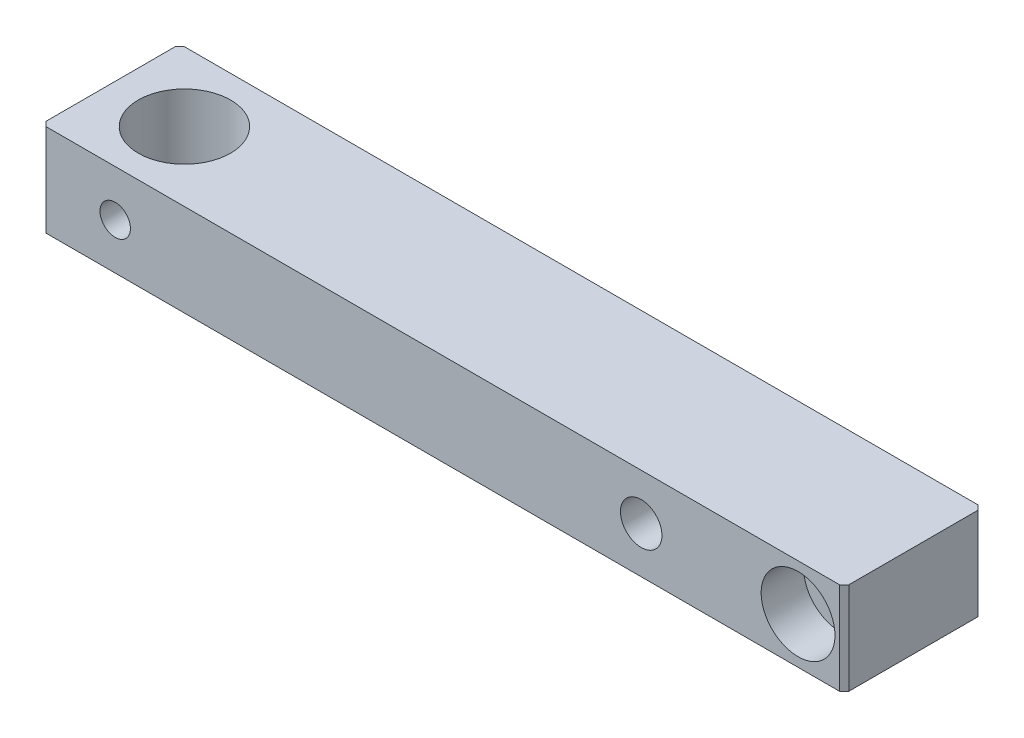
SolidWorks part; units mm, degrees
ref_plane "Front Plane" through (0, 0, 0) normal (0, 0, 1) x (1, 0, 0)
ref_plane "Top Plane" through (0, 0, 0) normal (0, 1, 0) x (1, 0, 0)
ref_plane "Right Plane" through (0, 0, 0) normal (1, 0, 0) x (0, 0, -1)
other "Configuration Table"
sketch "Sketch1" plane through (0, 0, 0) normal (0, 1, 0) x (1, 0, 0)
  line L1 (-43.5, 7.5) -> (43.5, 7.5)
  line L2 (-43.5, 7.5) -> (-43.5, -7.5)
  line L3 (-43.5, -7.5) -> (43.5, -7.5)
  line L4 (43.5, 7.5) -> (43.5, -7.5)
  line L5 (-43.5, 7.5) -> (43.5, -7.5) construction
  line L6 (-43.5, -7.5) -> (43.5, 7.5) construction
  point P0 (0, 0)
  dimension "D1" = 87
  dimension "D2" = 15
extrude "Boss-Extrude1" add sketch "Sketch1" along normal blind 10 contours L1 L4 L3 L2
sketch "Sketch2" plane through (0, 10, 0) normal (0, 1, 0) x (1, 0, 0)
  line L0 (-43.5, 7.5) -> (-43.5, -7.5) construction
  circle A0 centre (-35.5, 0) radius 5
  point P4 (-43.5, 0)
  dimension "D1" = 10
  dimension "D2" = 8
extrude "Cut-Extrude1" cut sketch "Sketch2" against normal through all
sketch "Sketch3" plane through (0, 0, -7.5) normal (0, 0, -1) x (-1, 0, 0)
  line L0 (-43.5, 10) -> (-43.5, 0) construction
  point P0 (-38.5, 5)
  point P3 (-43.5, 5)
  dimension "D1" = 5
sketch "Sketch5" plane through (0, 0, -7.5) normal (0, 0, -1) x (-1, 0, 0)
  line L0 (-43.5, 10) -> (-43.5, 0) construction
  point P0 (-21.5, 5)
  point P3 (-43.5, 5)
  dimension "D1" = 22
hole_wizard "Ø4.5 (4.5) Diameter Hole2" positions "Sketch5" profile "Sketch6" hole size "Ø4.5" standard "GB" end condition through all
sketch "Sketch6" plane through (21.5, 5, -7.5) normal (1, 0, 0) x (0, 1, 0)
  line L0 (0, 0) -> (0, 15)
  line L1 (0, 15) -> (2.25, 15)
  line L2 (2.25, 15) -> (2.25, 0)
  line L5 (2.25, 0) -> (0, 0)
  line L11 (0, -6.35) -> (0, 107.95) construction
  dimension "通孔孔直径" = 4.5
  dimension "通孔孔深度" = 15
sketch "Sketch7" plane through (0, 0, 7.5) normal (0, 0, 1) x (1, 0, 0)
  point P0 (38.5, 5)
hole_wizard "CBORE for M4 Slotted cheese head screws2" positions "Sketch7" profile "Sketch9" counterbore size "M4" standard "GB" end condition through all
sketch "Sketch9" plane through (38.5, 5, 7.5) normal (1, 0, 0) x (0, -1, 0)
  line L0 (0, 0) -> (0, 15)
  line L1 (0, 15) -> (2.25, 15)
  line L3 (2.25, 15) -> (2.25, 4.6)
  line L4 (2.25, 4.6) -> (4, 4.6)
  line L5 (4, 4.6) -> (4, 0)
  line L7 (4, 0) -> (0, 0)
  line L11 (0, -6.35) -> (0, 107.95) construction
  dimension "通孔孔直径" = 4.5
  dimension "通孔孔深度" = 15
  dimension "柱形沉头孔直径" = 8
  dimension "柱形沉头孔深度" = 4.6
chamfer "Chamfer1" distance 0.5 angle 45 4 edges at (43.5, 5, -7.5) (43.5, 5, 7.5) (-43.5, 5, -7.5) (-43.5, 5, 7.5)
sketch "Sketch10" plane through (0, 0, 7.5) normal (0, 0, 1) x (1, 0, 0)
  line L0 (-43, 10) -> (43, 10) construction
  line L1 (-43.5, 0) -> (-43.5, 10) construction
  point P0 (-35.5, 5)
  dimension "D1" = 5
  dimension "D2" = 8
hole_wizard "M4 Tapped Hole2" positions "Sketch10" profile "Sketch11" tap size "M4" standard "GB"
sketch "Sketch11" plane through (-35.5, 5, 7.5) normal (1, 0, 0) x (0, -1, 0)
  line L0 (0, 0) -> (0, 8.9914)
  line L1 (0, 8.9914) -> (1.65, 8)
  line L2 (1.65, 8) -> (1.65, 0)
  line L5 (1.65, 0) -> (0, 0)
  line L10 (0, 8.9914) -> (-1.65, 8) construction
  line L11 (0, -6.35) -> (0, 107.95) construction
  dimension "螺纹孔钻头直径" = 3.3
  dimension "螺纹孔钻头深度" = 8
  dimension "导头角度" = 118
cosmetic thread "Cosmetic thread 2" parameters "D1"=8, "D2"=4
